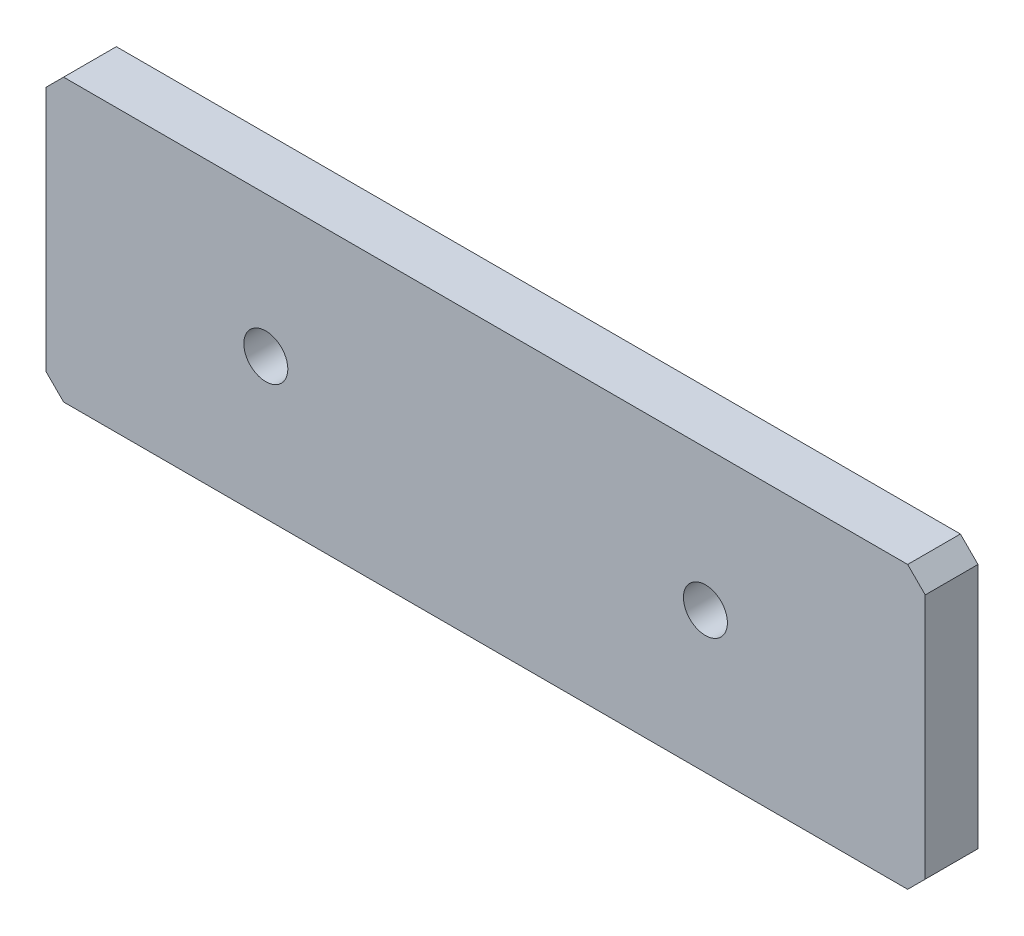
from build123d import *

# Parameters (mm, degrees)
SKETCH_1_W         = 50
SKETCH_1_H         = 16
EXTRUDE_1_DEPTH    = 1.5
HOLE_WIZARD_M3_1_D = 2.5
CHAMFER_1_SIZE     = 1


with BuildPart() as part:
    # 草图1 → 凸台-拉伸1 (new, symmetric)
    with BuildSketch(Plane.XY):
        Rectangle(SKETCH_1_W, SKETCH_1_H)
    extrude(amount=EXTRUDE_1_DEPTH, both=True)

    # M3 螺纹孔1 (through all)
    with Locations(Plane(origin=(0, 0, -1.5), x_dir=(-1, 0, 0), z_dir=(0, 0, -1))):
        with Locations((12.5, 0), (-12.5, 0)):
            Hole(HOLE_WIZARD_M3_1_D / 2)

    # 倒角1
    chamfer_1_edges = [part.edges().sort_by_distance(p)[0] for p in [
        (25, -8, 0),
        (-25, -8, 0),
        (-25, 8, 0),
        (25, 8, 0),
    ]]
    chamfer(chamfer_1_edges, length=CHAMFER_1_SIZE)


solid = part.part
